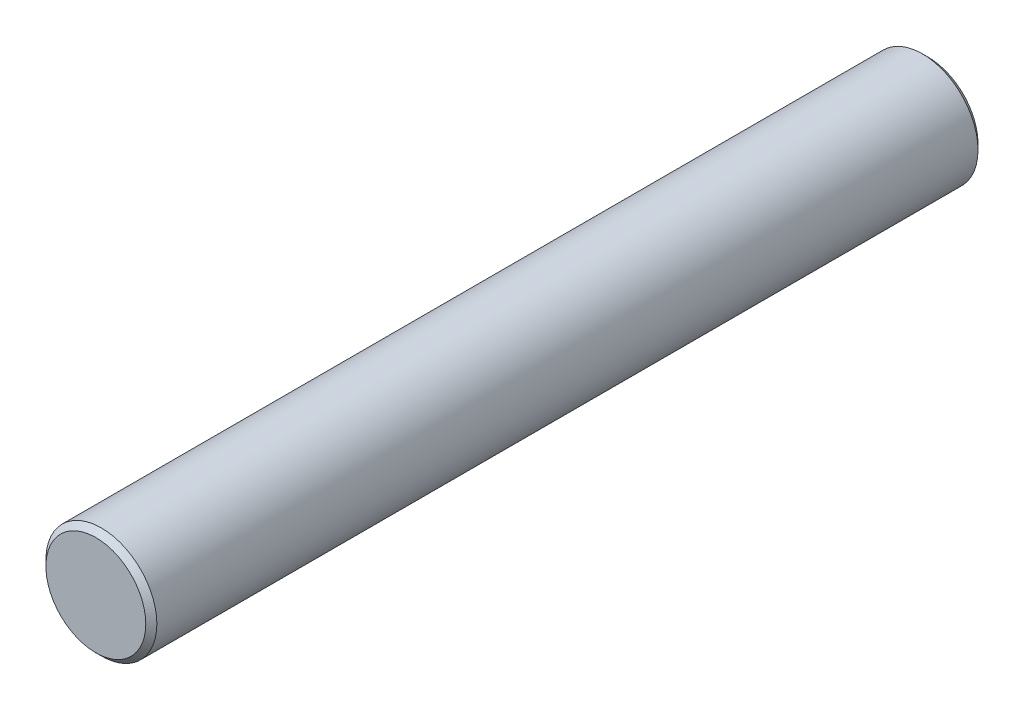
from build123d import *

# Parameters (mm, degrees)
SKETCH1_R           = 10
BOSS_EXTRUDE1_DEPTH = 150
CHAMFER1_SIZE       = 1


with BuildPart() as part:
    # Sketch1 → Boss-Extrude1 (new body)
    with BuildSketch(Plane.XY):
        Circle(SKETCH1_R)
    extrude(amount=-BOSS_EXTRUDE1_DEPTH)

    # Chamfer1
    chamfer1_edges = [part.edges().sort_by_distance(p)[0] for p in [
        (-10, 0, 0),
        (-10, 0, -150),
    ]]
    chamfer(chamfer1_edges, length=CHAMFER1_SIZE)


solid = part.part
